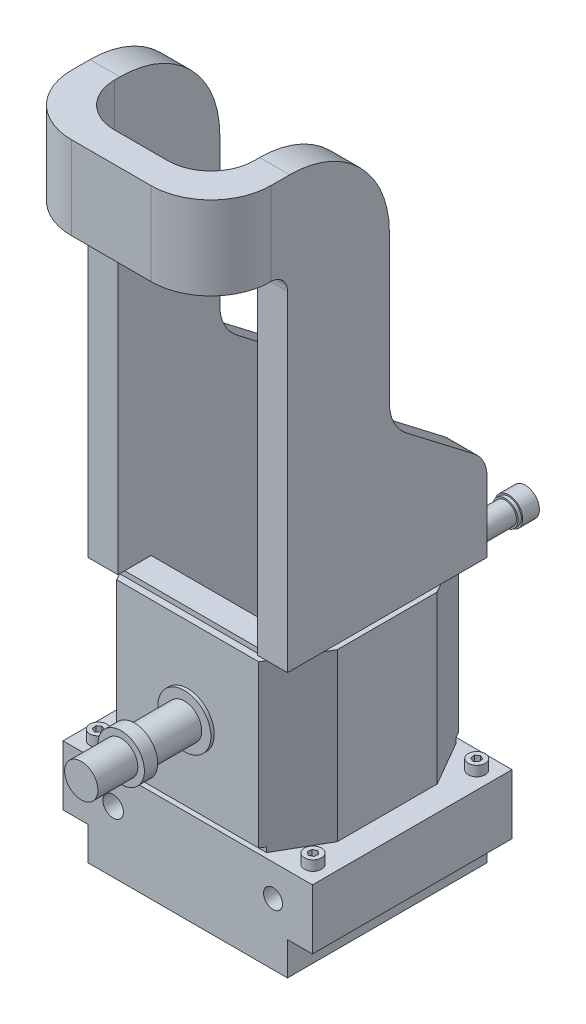
from build123d import *
from OCP.BRepFilletAPI import BRepFilletAPI_MakeChamfer

# Parameters (mm, degrees)
SKETCH1_W               = 60
SKETCH1_H               = 60
SKETCH1_W_2             = 40
SKETCH1_H_2             = 40
BOSS_EXTRUDE1_DEPTH     = 10
SKETCH2_W               = 75
SKETCH2_H               = 60
BOSS_EXTRUDE2_DEPTH     = 18
SKETCH4_W               = 60
SKETCH4_H               = 60
BOSS_EXTRUDE3_DEPTH     = 50
CHAMFER1_SIZE           = 15
CHAMFER1_SIZE2          = 8.660254038
CHAMFER2_SIZE           = 15
CHAMFER2_SIZE2          = 8.660254038
SKETCH5_W               = 30.45005041
SKETCH5_H               = 22.37154602
CUT_EXTRUDE1_DEPTH      = 20
CUT_EXTRUDE2_DEPTH      = 1.5
SKETCH7_R               = 2.547515883
BOSS_EXTRUDE4_DEPTH     = 3
MIRROR4_COPY_1_SKETCH_R = 2.547515883
MIRROR4_COPY_1_DEPTH    = 3
CUT_EXTRUDE3_REACH      = 107.31
SKETCH8_R               = 2.85561841
SKETCH8_R_2             = 3.077002641
SKETCH10_W              = 42
SKETCH10_H              = 40
CUT_EXTRUDE4_DEPTH      = 40
BOSS_EXTRUDE5_DEPTH     = 9
SKETCH12_W              = 56.09463004
SKETCH12_H              = 55.909804242
SKETCH12_W_2            = 42
SKETCH12_H_2            = 40
BOSS_EXTRUDE6_DEPTH     = 1.5
BOSS_EXTRUDE7_DEPTH     = 25
FILLET1_R               = 18
FILLET2_R               = 13
FILLET3_R               = 13
FILLET4_R               = 10
FILLET6_R               = 5
FILLET7_R               = 30
SKETCH14_R              = 3.332988603
SKETCH14_R_2            = 3.433487648
BOSS_EXTRUDE8_DEPTH     = 10
SKETCH15_R              = 3.805352351
SKETCH15_R_2            = 3.956911339
BOSS_EXTRUDE9_DEPTH     = 1
SKETCH16_R              = 4.230629521
SKETCH16_R_2            = 4.413958077
BOSS_EXTRUDE10_DEPTH    = 5
CUT_EXTRUDE5_DEPTH      = 3
SKETCH18_R              = 7.978631378
BOSS_EXTRUDE11_DEPTH    = 1
SKETCH19_R              = 5.221147189
BOSS_EXTRUDE12_DEPTH    = 15
SKETCH20_R              = 6.98705533
BOSS_EXTRUDE13_DEPTH    = 4
SKETCH21_R              = 5.009815996
BOSS_EXTRUDE14_DEPTH    = 12
SKETCH22_R              = 4.866265591
BOSS_EXTRUDE15_DEPTH    = 12
SKETCH23_R              = 6.441420435
BOSS_EXTRUDE16_DEPTH    = 6
SKETCH24_R              = 3.62644416
BOSS_EXTRUDE17_DEPTH    = 6


with BuildPart() as part:
    # Sketch1 → Boss-Extrude1 (new body)
    with BuildSketch(Plane(origin=(0, 0, 0), x_dir=(1, 0, 0), z_dir=(0, 1, 0))):
        Rectangle(SKETCH1_W, SKETCH1_H)
        Rectangle(SKETCH1_W_2, SKETCH1_H_2, mode=Mode.SUBTRACT)
    extrude(amount=BOSS_EXTRUDE1_DEPTH)

    # Sketch2 → Boss-Extrude2 (add)
    with BuildSketch(Plane(origin=(0, 10, 0), x_dir=(1, 0, 0), z_dir=(0, 1, 0))):
        Rectangle(SKETCH2_W, SKETCH2_H)
    extrude(amount=BOSS_EXTRUDE2_DEPTH)

    # Sketch4 → Boss-Extrude3 (add)
    with BuildSketch(Plane(origin=(0, 28, 0), x_dir=(1, 0, 0), z_dir=(0, 1, 0))):
        Rectangle(SKETCH4_W, SKETCH4_H)
    extrude(amount=BOSS_EXTRUDE3_DEPTH)

    # Chamfer1: one chamfer whose edges measure the first distance from different faces: ONE call of the kernel's chamfer builder (chamfer() names one face for all edges)
    chamfer1_edges_1 = [part.edges().sort_by_distance(p)[0] for p in [
        (-30, 53, 30),
    ]]
    chamfer1_side_1 = [part.faces().sort_by_distance(p)[0] for p in [
        (-30, 53, 0),
    ]]
    chamfer1_edges_2 = [part.edges().sort_by_distance(p)[0] for p in [
        (30, 53, -30),
    ]]
    chamfer1_side_2 = [part.faces().sort_by_distance(p)[0] for p in [
        (30, 53, 0),
    ]]
    chamfer1 = BRepFilletAPI_MakeChamfer(part.part.solid().wrapped)
    for e in chamfer1_edges_1:
        chamfer1.Add(CHAMFER1_SIZE, CHAMFER1_SIZE2, e.wrapped, chamfer1_side_1[0].wrapped)  # the first distance lies on this face
    for e in chamfer1_edges_2:
        chamfer1.Add(CHAMFER1_SIZE, CHAMFER1_SIZE2, e.wrapped, chamfer1_side_2[0].wrapped)  # the first distance lies on this face
    add(Compound.cast(chamfer1.Shape()), mode=Mode.REPLACE)

    # Chamfer2: one chamfer whose edges measure the first distance from different faces: ONE call of the kernel's chamfer builder (chamfer() names one face for all edges)
    chamfer2_edges_1 = [part.edges().sort_by_distance(p)[0] for p in [
        (-30, 53, -30),
    ]]
    chamfer2_side_1 = [part.faces().sort_by_distance(p)[0] for p in [
        (-30, 53, -7.5),
    ]]
    chamfer2_edges_2 = [part.edges().sort_by_distance(p)[0] for p in [
        (30, 53, 30),
    ]]
    chamfer2_side_2 = [part.faces().sort_by_distance(p)[0] for p in [
        (30, 53, 7.5),
    ]]
    chamfer2 = BRepFilletAPI_MakeChamfer(part.part.solid().wrapped)
    for e in chamfer2_edges_1:
        chamfer2.Add(CHAMFER2_SIZE, CHAMFER2_SIZE2, e.wrapped, chamfer2_side_1[0].wrapped)  # the first distance lies on this face
    for e in chamfer2_edges_2:
        chamfer2.Add(CHAMFER2_SIZE, CHAMFER2_SIZE2, e.wrapped, chamfer2_side_2[0].wrapped)  # the first distance lies on this face
    add(Compound.cast(chamfer2.Shape()), mode=Mode.REPLACE)

    # Sketch5 → Cut-Extrude1 (cut)
    with BuildSketch(Plane(origin=(0, 0, -30), x_dir=(-1, 0, 0), z_dir=(0, 0, -1))):
        with Locations((0, 59.769606645)):
            Rectangle(SKETCH5_W, SKETCH5_H)
    extrude(amount=-CUT_EXTRUDE1_DEPTH, mode=Mode.SUBTRACT)

    # Sketch6 → Cut-Extrude2 (cut)
    with BuildSketch(Plane(origin=(0, 28, 0), x_dir=(1, 0, 0), z_dir=(0, 1, 0))):
        Polygon((-24.812863535, 28.5), (23.79632164, 28.5), (23.79632164, 32.381341782), (-26.938360226, 32.381341782), align=None)
        Polygon((-25.87561188, -28.5), (26.568708627, -28.5), (25.367340933, -32.196515983), (-25.87561188, -32.196515983), align=None)
    extrude(amount=CUT_EXTRUDE2_DEPTH, mode=Mode.SUBTRACT)

    # Sketch7 → Boss-Extrude4 (add)
    with BuildSketch(Plane(origin=(0, 28, 0), x_dir=(1, 0, 0), z_dir=(0, 1, 0))):
        with Locations(Location((32.275998147, 24.610235837, 0), (0, 0, 270))):
            Circle(SKETCH7_R)
        Polygon((33.484611692, 24.093844051), (33.327513325, 25.398729977), (32.118899781, 25.915121764), (31.067384603, 25.126627624), (31.22448297, 23.821741698), (32.433096514, 23.305349911), align=None, mode=Mode.SUBTRACT)
    boss_extrude4 = extrude(amount=BOSS_EXTRUDE4_DEPTH)

    # Mirror3: Boss-Extrude4 across plane
    add(boss_extrude4.mirror(Plane(origin=(0, 0, 0), x_dir=(0, 0, 1), z_dir=(1, 0, 0))))

    # Mirror4: Boss-Extrude4 across plane
    add(boss_extrude4.mirror(Plane.XY))

    # Mirror4 copy 1 sketch → Mirror4 copy 1 (add)
    with BuildSketch(Plane(origin=(0, 28, 0), x_dir=(-1, 0, 0), z_dir=(0, 1, 0))):
        with Locations(Location((32.275998147, 24.610235837, 0), (0, 0, 270))):
            Circle(MIRROR4_COPY_1_SKETCH_R)
        Polygon((33.484611692, 24.093844051), (33.327513325, 25.398729977), (32.118899781, 25.915121764), (31.067384603, 25.126627624), (31.22448297, 23.821741698), (32.433096514, 23.305349911), align=None, mode=Mode.SUBTRACT)
    extrude(amount=MIRROR4_COPY_1_DEPTH)

    # Sketch8 → Cut-Extrude3 (cut, up to next)
    with BuildSketch(Plane(origin=(0, 0, -30), x_dir=(-1, 0, 0), z_dir=(0, 0, -1)), mode=Mode.PRIVATE) as cut_extrude3_sk1:
        with Locations((-25.649200277, 18.51668081)):
            Circle(SKETCH8_R)
    cut_extrude3_tool1 = extrude(cut_extrude3_sk1.sketch, amount=-CUT_EXTRUDE3_REACH, mode=Mode.PRIVATE) & part.part
    # Sketch8 → Cut-Extrude3 (cut, up to next)
    with BuildSketch(Plane(origin=(0, 0, -30), x_dir=(-1, 0, 0), z_dir=(0, 0, -1)), mode=Mode.PRIVATE) as cut_extrude3_sk2:
        with Locations((22.405507501, 18.51668081)):
            Circle(SKETCH8_R_2)
    cut_extrude3_tool2 = extrude(cut_extrude3_sk2.sketch, amount=-CUT_EXTRUDE3_REACH, mode=Mode.PRIVATE) & part.part
    add(cut_extrude3_tool1.solids().sort_by_distance((25.6492, 18.516681, -30))[0], mode=Mode.SUBTRACT)
    add(cut_extrude3_tool2.solids().sort_by_distance((-22.405508, 18.516681, -30))[0], mode=Mode.SUBTRACT)

    # Sketch10 → Cut-Extrude4 (cut)
    with BuildSketch(Plane(origin=(0, 78, 0), x_dir=(1, 0, 0), z_dir=(0, 1, 0))):
        Rectangle(SKETCH10_W, SKETCH10_H)
    extrude(amount=-CUT_EXTRUDE4_DEPTH, mode=Mode.SUBTRACT)



with BuildPart() as body_2:
    # Sketch11 → Boss-Extrude5 (new body)
    with BuildSketch(Plane(origin=(30, 0, 0), x_dir=(0, 0, -1), z_dir=(1, 0, 0))):
        Polygon((-30, 79.5), (-30, 183.792470171), (0.640507311, 183.792470171), (0.640507311, 127.940232676), (30, 105.408087073), (30, 79.5), align=None)
    boss_extrude5 = extrude(amount=-BOSS_EXTRUDE5_DEPTH)


with BuildPart() as part_1:
    add(part.part)

    add(body_2.part)  # Boss-Extrude6 merges body 2
    # Sketch12 → Boss-Extrude6 (add)
    with BuildSketch(Plane(origin=(0, 78, 0), x_dir=(1, 0, 0), z_dir=(0, 1, 0))):
        Rectangle(SKETCH12_W, SKETCH12_H)
        Rectangle(SKETCH12_W_2, SKETCH12_H_2, mode=Mode.SUBTRACT)
    extrude(amount=BOSS_EXTRUDE6_DEPTH)

    # Mirror5: Boss-Extrude5 across plane
    add(boss_extrude5.mirror(Plane(origin=(0, 0, 0), x_dir=(0, 0, 1), z_dir=(1, 0, 0))))

    # Sketch13 → Boss-Extrude7 (add)
    with BuildSketch(Plane(origin=(0, 183.792470171, 0), x_dir=(1, 0, 0), z_dir=(0, 1, 0))):
        Polygon((-30, 0.640507311), (-21, 0.640507311), (-21, -30), (-21, -44), (21, -44), (21, -30), (21, 0.640507311), (30, 0.640507311), (30, -53), (-30, -53), align=None)
    extrude(amount=BOSS_EXTRUDE7_DEPTH)

    # Fillet1
    fillet1_edges = [part_1.edges().sort_by_distance(p)[0] for p in [
        (-30, 196.292470171, 53),
        (30, 196.292470171, 53),
    ]]
    fillet(fillet1_edges, radius=FILLET1_R)

    # Fillet2
    fillet2_edges = [part_1.edges().sort_by_distance(p)[0] for p in [
        (21, 196.292470171, 44),
        (-21, 196.292470171, 44),
    ]]
    fillet(fillet2_edges, radius=FILLET2_R)

    # Fillet3
    fillet3_edges = [part_1.edges().sort_by_distance(p)[0] for p in [
        (25.5, 127.940232676, -0.640507311),
        (-25.5, 127.940232676, -0.640507311),
    ]]
    fillet(fillet3_edges, radius=FILLET3_R)

    # Fillet4
    fillet4_edges = [part_1.edges().sort_by_distance(p)[0] for p in [
        (25.5, 105.408087073, -30),
        (-25.5, 105.408087073, -30),
    ]]
    fillet(fillet4_edges, radius=FILLET4_R)

    # Fillet6
    fillet6_edges = [part_1.edges().sort_by_distance(p)[0] for p in [
        (-25.5, 183.792470171, 30),
        (25.5, 183.792470171, 30),
    ]]
    fillet(fillet6_edges, radius=FILLET6_R)

    # Fillet7
    fillet7_edges = [part_1.edges().sort_by_distance(p)[0] for p in [
        (25.5, 208.792470171, -0.640507311),
        (-25.5, 208.792470171, -0.640507311),
    ]]
    fillet(fillet7_edges, radius=FILLET7_R)

    # Sketch14 → Boss-Extrude8 (add)
    with BuildSketch(Plane(origin=(0, 0, -30), x_dir=(-1, 0, 0), z_dir=(0, 0, -1))):
        with Locations((-25.5, 83.812817652)):
            Circle(SKETCH14_R)
        with Locations(Location((25.669245773, 83.812817652, 0), (0, 0, 180))):
            Circle(SKETCH14_R_2)
    extrude(amount=BOSS_EXTRUDE8_DEPTH)

    # Sketch15 → Boss-Extrude9 (add)
    with BuildSketch(Plane(origin=(0, 0, -40), x_dir=(-1, 0, 0), z_dir=(0, 0, -1))):
        with Locations((-25.5, 83.812817652)):
            Circle(SKETCH15_R)
        with Locations((25.669245773, 83.812817652)):
            Circle(SKETCH15_R_2)
    extrude(amount=BOSS_EXTRUDE9_DEPTH)

    # Sketch16 → Boss-Extrude10 (add)
    with BuildSketch(Plane(origin=(0, 0, -41), x_dir=(-1, 0, 0), z_dir=(0, 0, -1))):
        with Locations((-25.5, 83.812817652)):
            Circle(SKETCH16_R)
        with Locations((25.669245773, 83.812817652)):
            Circle(SKETCH16_R_2)
    extrude(amount=BOSS_EXTRUDE10_DEPTH)

    # Sketch17 → Cut-Extrude5 (cut)
    with BuildSketch(Plane(origin=(0, 0, -46), x_dir=(-1, 0, 0), z_dir=(0, 0, -1))):
        Polygon((-23.5769975, 82.557550901), (-23.451405856, 84.850553293), (-25.374408356, 86.105820043), (-27.4230025, 85.068084402), (-27.548594144, 82.77508201), (-25.625591644, 81.51981526), align=None)
        Polygon((27.647879806, 82.557550901), (27.745655684, 84.898731614), (25.767021651, 86.153998364), (23.690611741, 85.068084402), (23.592835863, 82.72690369), (25.571469895, 81.47163694), align=None)
    extrude(amount=-CUT_EXTRUDE5_DEPTH, mode=Mode.SUBTRACT)

    # Sketch18 → Boss-Extrude11 (add)
    with BuildSketch(Plane.XY.offset(30)):
        with Locations((0, 52.396218425)):
            Circle(SKETCH18_R)
    extrude(amount=BOSS_EXTRUDE11_DEPTH)

    # Sketch19 → Boss-Extrude12 (add)
    with BuildSketch(Plane.XY.offset(31)):
        with Locations((0, 52.396218425)):
            Circle(SKETCH19_R)
    extrude(amount=BOSS_EXTRUDE12_DEPTH)

    # Sketch20 → Boss-Extrude13 (add)
    with BuildSketch(Plane.XY.offset(46)):
        with Locations((0, 52.396218425)):
            Circle(SKETCH20_R)
    extrude(amount=BOSS_EXTRUDE13_DEPTH)

    # Sketch21 → Boss-Extrude14 (add)
    with BuildSketch(Plane.XY.offset(50)):
        with Locations((0, 52.396218425)):
            Circle(SKETCH21_R)
    extrude(amount=BOSS_EXTRUDE14_DEPTH)

    # Sketch22 → Boss-Extrude15 (add)
    with BuildSketch(Plane(origin=(0, 0, 20), x_dir=(-1, 0, 0), z_dir=(0, 0, -1))):
        with Locations(Location((0, 59.519830647, 0), (0, 0, 180))):
            Circle(SKETCH22_R)
    extrude(amount=BOSS_EXTRUDE15_DEPTH)

    # Sketch23 → Boss-Extrude16 (add)
    with BuildSketch(Plane(origin=(0, 0, 8), x_dir=(-1, 0, 0), z_dir=(0, 0, -1))):
        with Locations((0, 59.519830647)):
            Circle(SKETCH23_R)
        Polygon((2.679035332, 57.597233825), (3.004535355, 60.878644891), (0.325500023, 62.801241713), (-2.679035332, 61.442427469), (-3.004535355, 58.161016403), (-0.325500023, 56.238419581), align=None, mode=Mode.SUBTRACT)
    extrude(amount=BOSS_EXTRUDE16_DEPTH)

    # Sketch24 → Boss-Extrude17 (add)
    with BuildSketch(Plane(origin=(0, 0, -30), x_dir=(-1, 0, 0), z_dir=(0, 0, -1))):
        with Locations(Location((0, 38.12935067, 0), (0, 0, 180))):
            Circle(SKETCH24_R)
    extrude(amount=BOSS_EXTRUDE17_DEPTH)


solid = part_1.part
